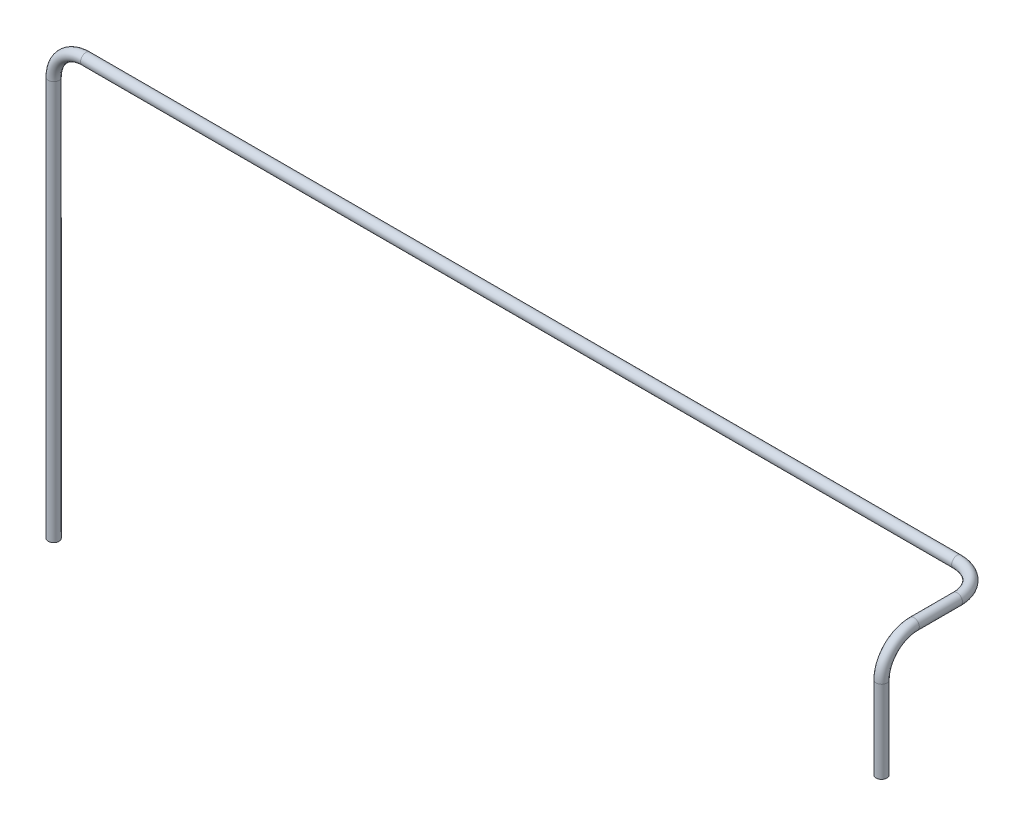
from build123d import *

# Parameters (mm, degrees)
SWEEP_THIN1_PROFILE_R   = 10
SWEEP_THIN1_PROFILE_R_2 = 5


with BuildPart() as part:
    # Sweep-Thin1: sweep along a curve in space
    with BuildLine() as sweep_thin1_path:
        Line((2400, 1637.292385154, -1100), (2400, 1790.038439201, -1100))
        ThreePointArc((2400, 1790.038439201, -1100), (2400, 1832.464846073, -1117.573593129), (2400, 1850.038439201, -1160))
        Line((2400, 1850.038439201, -1160), (2400, 1850.038439201, -1240))
        ThreePointArc((2400, 1850.038439201, -1240), (2382.426406871, 1850.038439201, -1282.426406871), (2340, 1850.038439201, -1300))
        Line((2340, 1850.038439201, -1300), (725.34875551, 1850.038439201, -1300))
        ThreePointArc((725.34875551, 1850.038439201, -1300), (682.922348639, 1832.464846073, -1300), (665.34875551, 1790.038439201, -1300))
        Line((665.34875551, 1790.038439201, -1300), (665.34875551, 1050.038439201, -1300))
    # Sweep-Thin1 profile (on start of the path) → Sweep-Thin1 (sweep)
    with BuildSketch(Plane(origin=(2400, 1637.292385154, -1100), x_dir=(0, 0, 1), z_dir=(0, 1, 0))):
        Circle(SWEEP_THIN1_PROFILE_R)
        Circle(SWEEP_THIN1_PROFILE_R_2, mode=Mode.SUBTRACT)
    sweep(path=sweep_thin1_path.line)


solid = part.part
